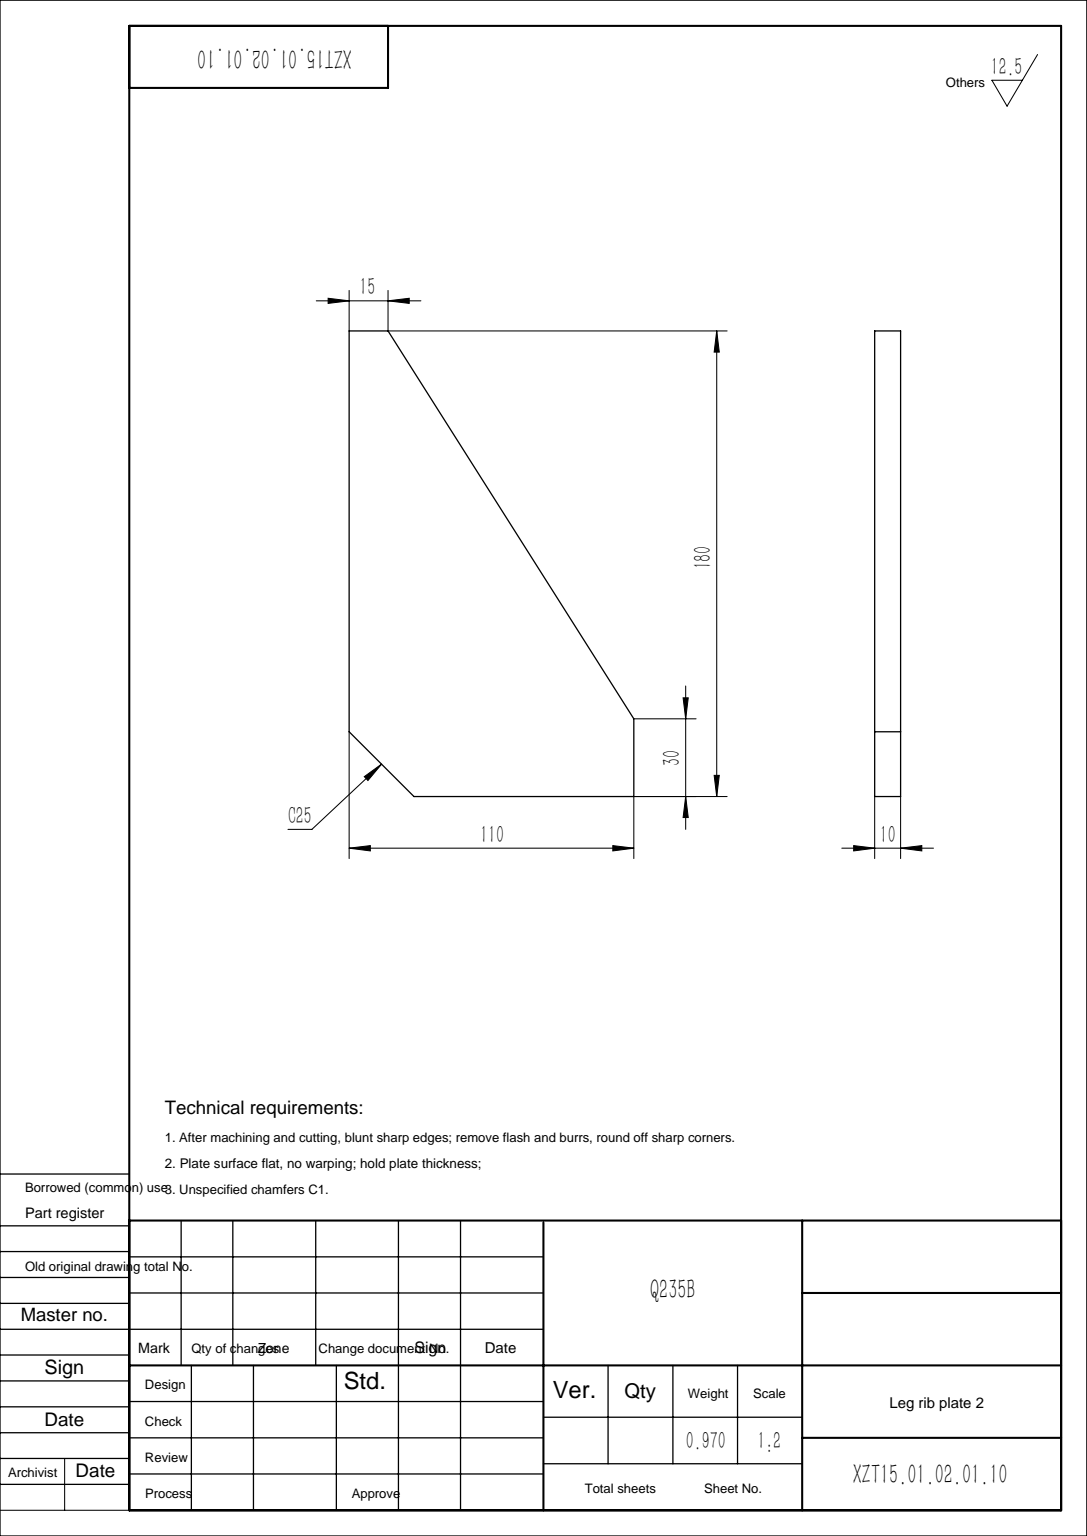
SolidWorks part; units mm, degrees
material "Q235B"
ref_plane "Front Plane" through (0, 0, 0) normal (0, 0, 1) x (1, 0, 0)
ref_plane "Top Plane" through (0, 0, 0) normal (0, 1, 0) x (1, 0, 0)
ref_plane "Right Plane" through (0, 0, 0) normal (1, 0, 0) x (0, 0, -1)
sketch "Sketch1" plane through (0, 0, 0) normal (0, 0, 1) x (1, 0, 0)
  line L0 (0, 0) -> (110, 0)
  line L1 (110, 0) -> (110, 30)
  line L2 (110, 30) -> (15, 180)
  line L3 (15, 180) -> (0, 180)
  line L4 (0, 180) -> (0, 0)
  dimension "D1" = 110
  dimension "D2" = 30
  dimension "D3" = 15
  dimension "D4" = 180
extrude "Boss-Extrude1" add sketch "Sketch1" along normal mid plane 10
chamfer "Chamfer1" distance 25 angle 45 1 edges at (0, 0, 0)
